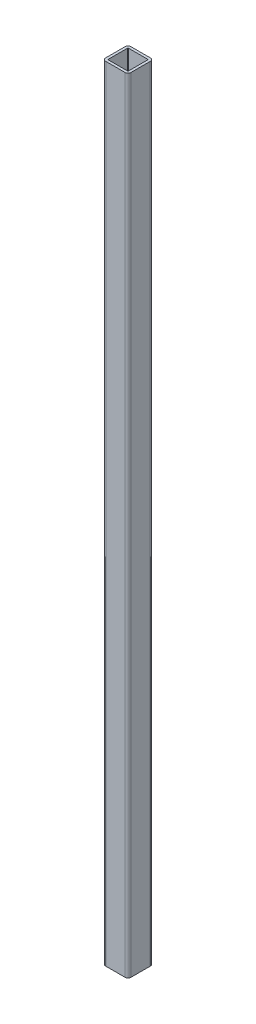
SolidWorks part; units mm, degrees
ref_plane "Front" through (0, 0, 0) normal (0, 0, 1) x (1, 0, 0)
ref_plane "Top" through (0, 0, 0) normal (0, 1, 0) x (1, 0, 0)
ref_plane "Right" through (0, 0, 0) normal (1, 0, 0) x (0, 0, -1)
sketch "草图1" plane through (0, 0, 0) normal (0, 1, 0) x (1, 0, 0)
  line L0 (-19, -20) -> (19, -20)
  line L1 (-19, -25) -> (19, -25)
  line L2 (-25, -19) -> (-25, 19)
  line L3 (-19, 25) -> (19, 25)
  line L4 (25, -19) -> (25, 19)
  line L5 (-25, -25) -> (25, 25) construction
  line L6 (-25, 25) -> (25, -25) construction
  line L7 (20, -19) -> (20, 19)
  line L8 (-19, 20) -> (19, 20)
  line L9 (-20, -19) -> (-20, 19)
  arc A0 (-19, -25) -> (-25, -19) centre (-19, -19) cw
  arc A1 (19, -25) -> (25, -19) centre (19, -19) ccw
  arc A2 (19, 25) -> (25, 19) centre (19, 19) cw
  arc A3 (-25, 19) -> (-19, 25) centre (-19, 19) cw
  arc A4 (19, -20) -> (20, -19) centre (19, -19) ccw
  arc A5 (19, 20) -> (20, 19) centre (19, 19) cw
  arc A6 (-20, 19) -> (-19, 20) centre (-19, 19) cw
  arc A7 (-19, -20) -> (-20, -19) centre (-19, -19) cw
  point P0 (0, 0)
  dimension "D3" = 6
  dimension "D1" = 50
  dimension "D2" = 50
  dimension "D4" = 5
extrude "凸台-拉伸1" add sketch "草图1" along normal blind 1550
